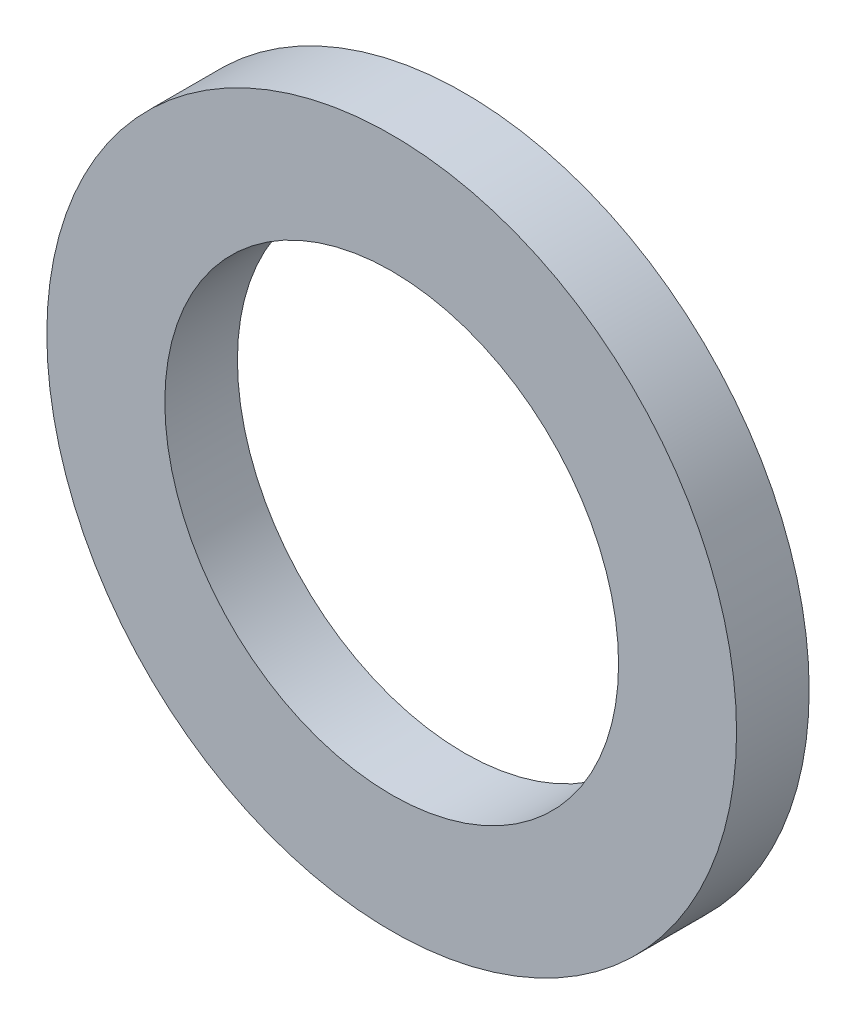
SolidWorks part; units mm, degrees
material "Q235B"
ref_plane "Front Plane" through (0, 0, 0) normal (0, 0, 1) x (1, 0, 0)
ref_plane "Top Plane" through (0, 0, 0) normal (0, 1, 0) x (1, 0, 0)
ref_plane "Right Plane" through (0, 0, 0) normal (1, 0, 0) x (0, 0, -1)
sketch "Sketch1" plane through (0, 0, 0) normal (0, 0, 1) x (1, 0, 0)
  circle A0 centre (0, 0) radius 19
  circle A1 centre (0, 0) radius 12.5
  dimension "d2" = 38
  dimension "d1" = 25
extrude "Extrude1" add sketch "Sketch1" along normal blind 4
